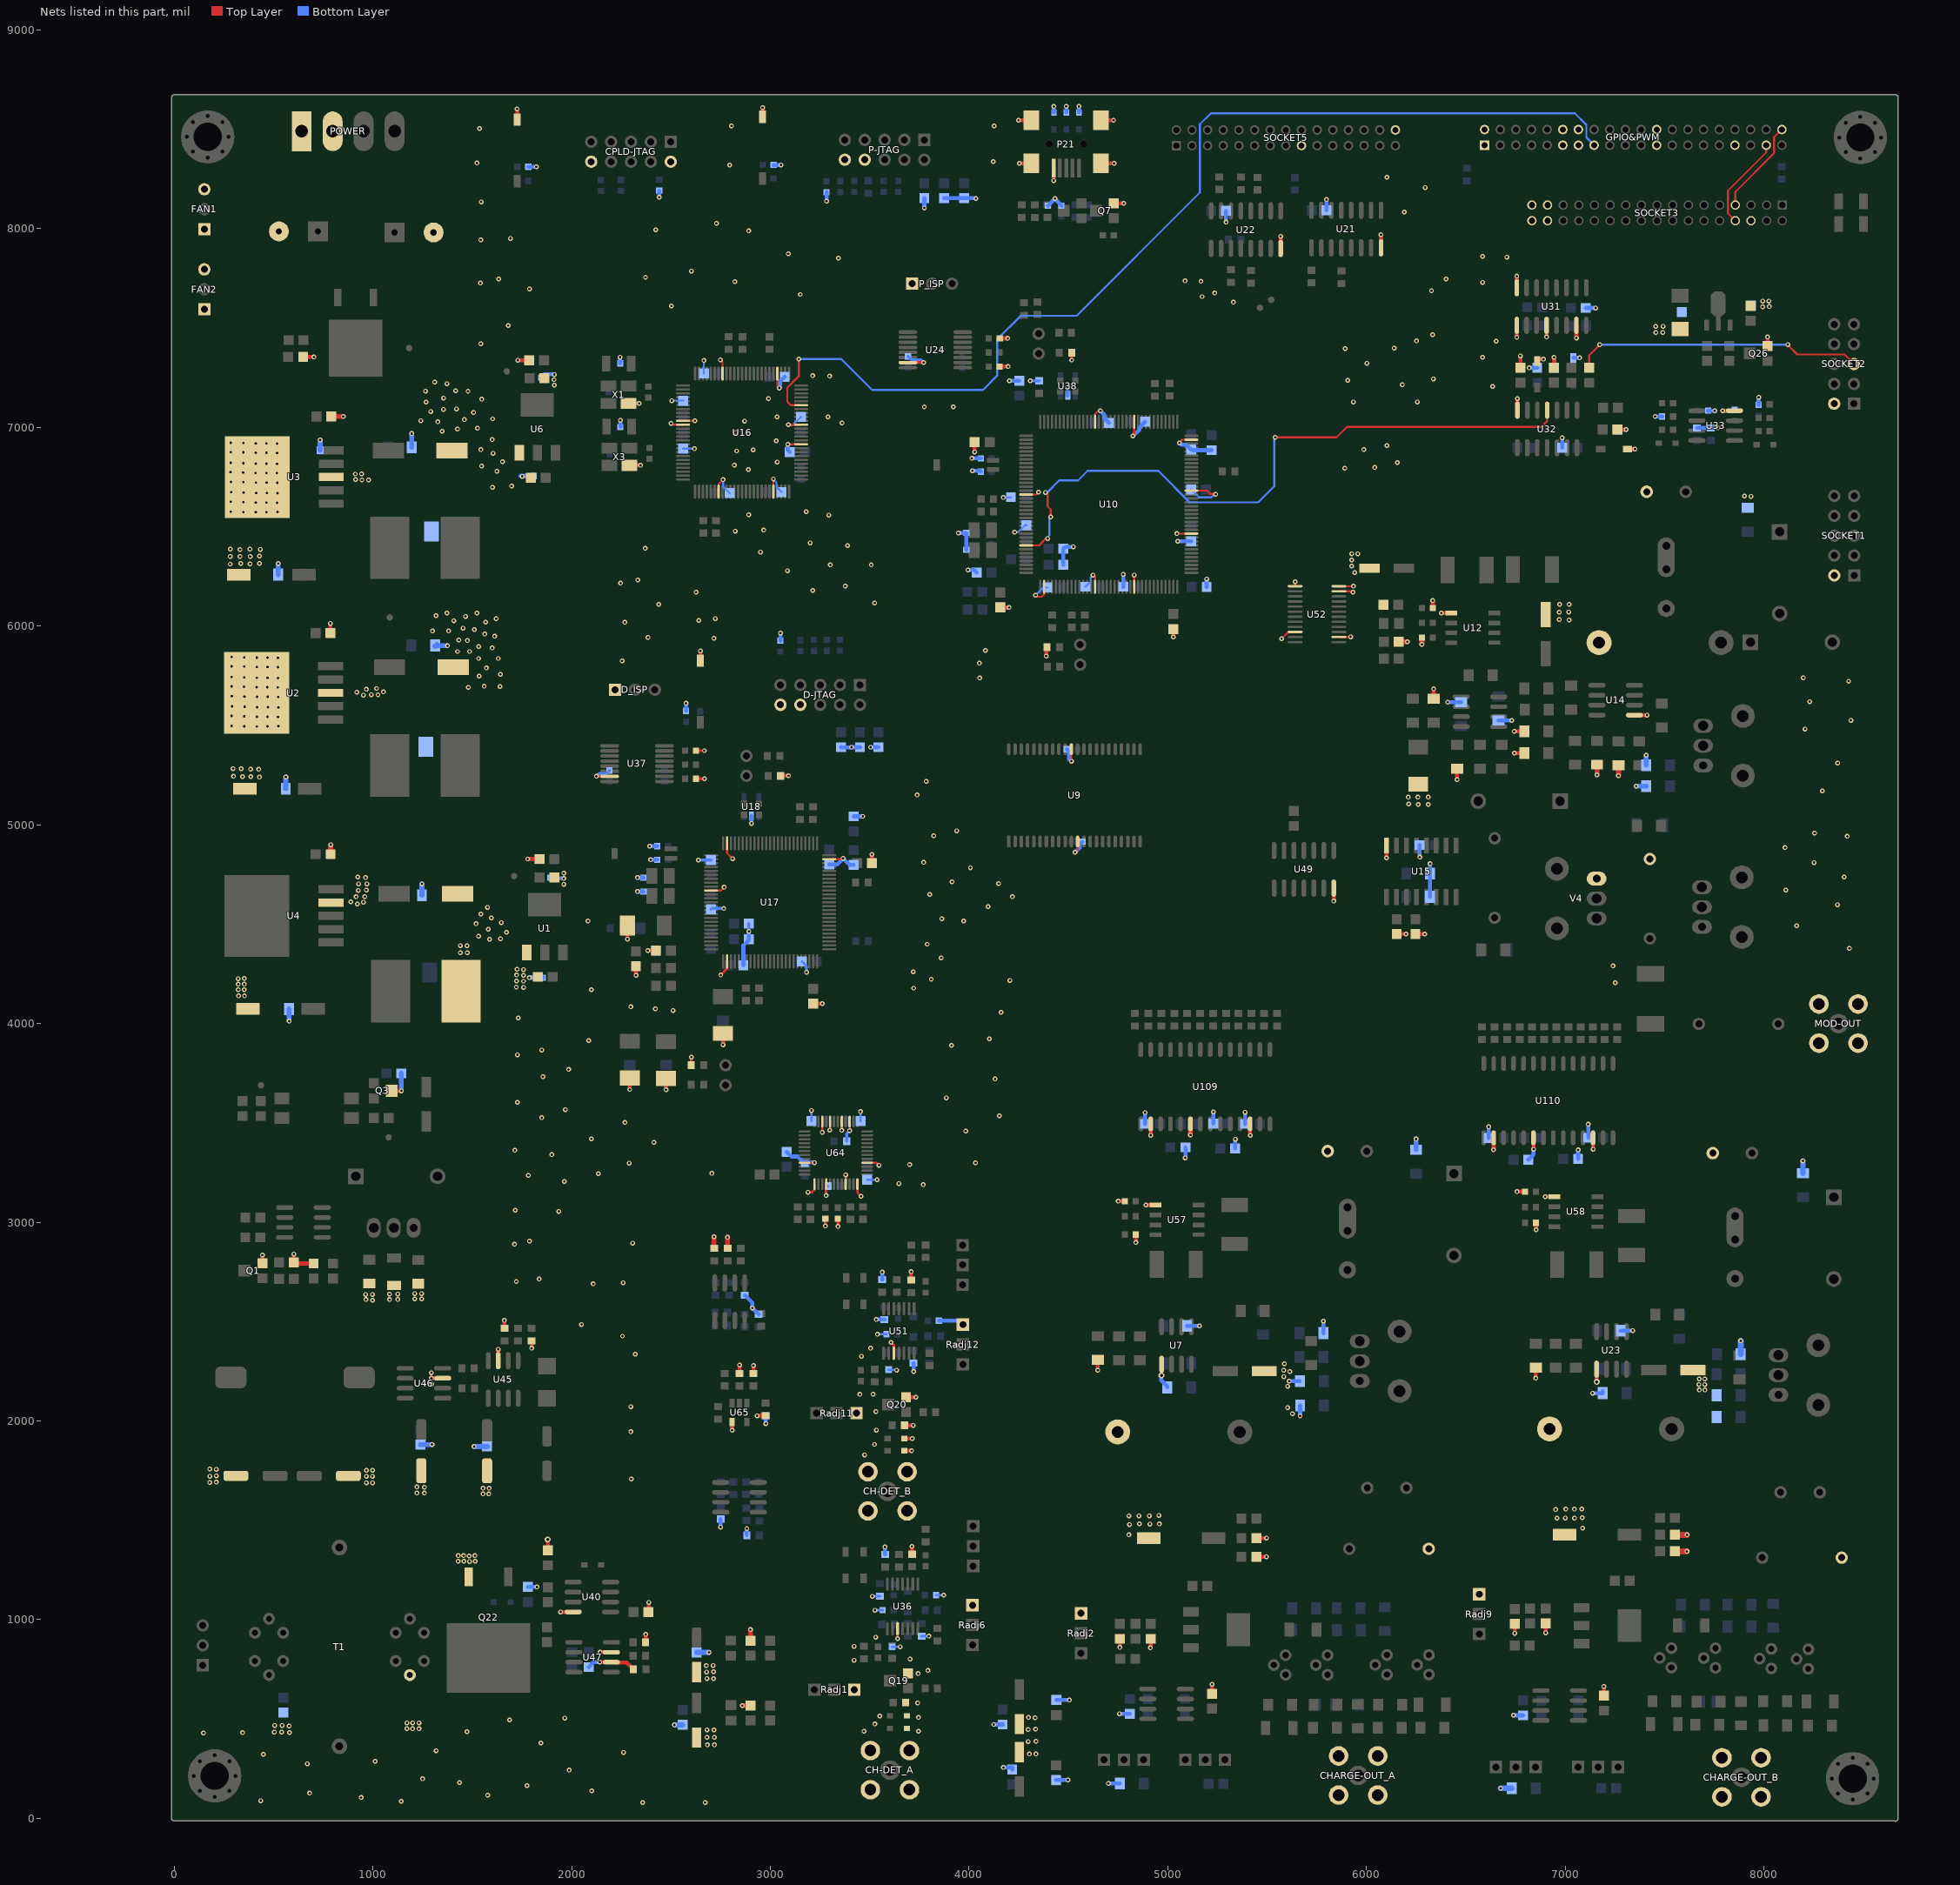
[diagram p0: the nets of this part, all layers, seen from the top]
# Altium PCB MISC82309.PcbDoc (part 8 of 14)
Units mil, origin at the board's own origin, x right, y up, seen from the top; angles counter-clockwise.
Board outline 8687.03 x 8687.86 mil, 4 copper layers (Top Layer, GND, POWER, Bottom Layer); 747 components, 583 nets, 2530 pads, 1834 vias.

## Via types
v1: diameter 24, hole 12, Top Layer to Bottom Layer, 1799 vias
v2: diameter 30, hole 15, Top Layer to Bottom Layer, 26 vias
v3: diameter 40, hole 20, Top Layer to Bottom Layer, 9 vias

## Nets (pads, with @x,y where several pads share a name; then routed paths per layer and width w, separated by ;. In a path a pad name is that pad's centre, name@x,y a point inside that pad or via, vN(x,y) a via of type N, cw(c..) or ccw(c..) an arc to the next point about the centre after c; other vN are vias at no path point) (continued)
GND: C1.1 C2.1 C3.2 C4.2 C5.2 C6.1 C7.1 C8.1 C9.2 C10.2 C11.2 C12.1 C13.1 C14.1 C15.2 C16.1 C18.1 C19.1 C20.1 C24.2 C25.2 C27.2 C28.2 C29.2 C31.2 C32.2 C33.1 C34.1 C35.1 C36.1 C37.1 C38.1 C39.1 C40.1 C41.1 C42.1 C45.2 C48.2 C49.2 C50.2 C51.2 C52.2 C53.2 C54.2 C55.1 C56.2 C57.2 C63.1 C64.1 C65.1 C66.1 C67.2 C68.2 C69.2 C70.1 C71.1 C72.1 C73.1 C74.1 C75.1 C78.2 C79.1 C80.1 C81.1 C82.1 C83.1 C84.1 C85.1 C86.1 C87.1 C88.1 C89.1 C90.1 C93.1 C94.1 C98.1 C99.1 C123.1 C124.1 C125.1 C126.1 C127.1 C128.1 C129.1 C130.1 C131.1 C132.1 C133.1 C134.1 C141.1 C142.1 C143.1 C146.1 C147.1 C148.1 C151.1 C153.2 C154.1 C155.2 C156.2 C157.2 C158.2 C159.1 C162.1 C164.1 C165.1 C167.2 C170.2 C171.2 C172.1 C173.1 C174.1 C175.1 C176.1 C179.1 C180.1 C181.1 C182.1 C183.1 C184.1 C188.1 C193.1 C195.1 C196.1 C197.1 C198.1 C199.1 C200.1 C201.1 C202.1 C210.1 C214.2 C215.2 C220.1 C221.1 C226.1 C227.1 C228.1 C230.1 C231.1 C232.1 C233.1 C240.1 C241.1 C242.1 C243.1 C244.1 C245.1 C246.1 C247.1 C248.1 C249.1 C250.1 C251.1 C252.1 C253.1 C254.1 C255.1 C256.2 C257.2 C263.2 C266.2 C267.2 C270.2 C271.2 C277.2 C278.2 C279.1 C280.1 C281.1 C283.2 C284.2 C285.1 C288.1 C292.2 C293.2 C317.2 C318.2 C364.1 C370.1 C373.1 C374.1 C411.1 C412.1 C413.1 C420.1 C421.1 C423.2 C424.1 C449.1 C506.2 C507.2 C599.2 CH-DET_A.2 CH-DET_B.2 CHARGE-OUT_A.M-1 CHARGE-OUT_A.M-2 CHARGE-OUT_A.M-3 CHARGE-OUT_A.M-4 CHARGE-OUT_B.M-1 CHARGE-OUT_B.M-2 CHARGE-OUT_B.M-3 CHARGE-OUT_B.M-4 CPLD-JTAG.2 CPLD-JTAG.10 CPLD_REST.1 D2.1 D3.1 D6.1 D14.1 D23.1 D24.1 D25.2 D26.1 D28.1 D29.1 D34.1 D35.1 D40.1 D46.1 D47.2 D52.1 D54.1 D55.2 D-JTAG.8 D-JTAG.10 D_ISP.1 D_REST.2 ESD23.2 ESD24.2 ESD25.2 FAN1.1 FAN1.3 FAN2.1 FAN2.3 GPIO&PWM.1 GPIO&PWM.2 GPIO&PWM.11 GPIO&PWM.12 GPIO&PWM.13 GPIO&PWM.14 GPIO&PWM.23 GPIO&PWM.24 GPIO&PWM.33 L4.2 LED1.2 LED2.2 LED3.2 LED4.1 LED5.2 LED6.2 MOD-OUT.2 P21.5 P21.6 P21.7 P21.8 P21.9 P-JTAG.8 P-JTAG.10 P_ISP.1 P_REST.2 POWER.1 POWER.2 Q1.2 Q3.3 Q7.2 Q19.2 Q20.2 Q22.3 Q26.2 R13.2 R15.2 R17.1 R22.2 R27.1 R28.1 R29.1 R33.1 R34.2 R39.1 R46.2 R48.1 R61.2 R62.2 R64.2 R65.2 R68.1 R74.1 R76.1 R79.1 R84.1 R85.1 R151.1 R157.1 R158.1 R168.1 R174.2 R190.1 R192.1 R194.1 R197.1 R217.2 R220.2 R221.1 R222.2 R269.2 R275.1 R286.1 R287.1 R292.1 R293.2 R294.1 R295.2 R313.1 R314.2 R315.1 R316.1 R318.2 R326.1 R328.1 R330.1 R333.1 R343.1 R374.2 R411.2 R417.2 R495.1 R496.1 R517.2 R521.2 R545.1 R546.1 R555.1 R591.1 R595.1 R599.1 Radj1.1 Radj2.3 Radj6.1 Radj9.3 Radj11.1 Radj12.1 SOCKET1.2 SOCKET2.2 SOCKET3.6 SOCKET3.31 SOCKET3.32 SOCKET3.33 SOCKET3.34 SOCKET5.17 SOCKET5.30 T1.3 TC2.1 TC3.1 U1.1 U2.3 U2.6 U3.3 U3.6 U4.4 U6.1 U7.5 U9.12 U9.34 U10.16 U10.38 U10.51 U10.61 U10.83 U10.94 U10.107 U10.120 U10.130 U12.1 U14.5 U15.16 U16.10 U16.11 U16.32 U16.46 U16.60 U16.65 U16.79 U16.93 U17.10 U17.27 U17.74 U17.99 U18.2 U21.8 U22.8 U23.5 U24.15 U31.8 U31.9 U31.12 U31.15 U32.7 U33.4 U36.3 U37.15 U38.2 U40.4 U45.3 U46.3 U47.2 U47.3 U49.7 U51.3 U52.2 U52.11 U52.12 U52.13 U52.22 U57.1 U58.1 U64.1 U64.4 U64.9 U64.12 U64.16 U64.27 U64.29 U64.32 U64.34 U64.45 U65.4 U109.16 U109.20 U109.26 U110.16 U110.20 U110.26 V1.1 V4.3 X1.2 X3.2 | length 17920.4
  Top Layer w10: v1(2501,7020) 2507.63,7013.37 U16.11@2560.76,7013.37 ; U16.10@2560.76,7033.06 v1(2620.06,7033.06) ; U17.10@2701.76,4669.06 2751.06,4669.06 v1(2768,4686) ; U16.32@2739.89,6676.76 2739.89,6714.89 v1(2762,6737) ; v1(2749,7339) 2759.57,7328.43 U16.93@2759.57,7271.24 ; U17.99@2782.46,4907.24 2782.46,4857.54 v1(2810,4830) ; U16.46@3015.48,6676.76 v1(3015.48,6740.48) ; U16.79@3035.17,7271.24 3035.17,7206.83 3044,7198 v1(3045,7198) ; v1(3088.06,6914.94) U16.60@3155.24,6914.94 ; v1(3090.63,7013.37) U16.65@3155.24,7013.37 ; U64.45@3172.52,3299.79 v1(3221.79,3299.79) ; U17.74@3296.24,4826.54 v1@3361.54,4826.54 ; U10.16@4287.65,6662.21 4338.21,6662.21 v1(4350,6674) ; v1(4335,6155) 4342,6148 4365,6148 4378.2,6161.2 U10.38@4378.2,6197.65 ; v1(4514.96,5320.04) U9.34@4514.96,5380.57 ; v1(4533,4862) 4532,4862 4546.46,4876.46 U9.12@4546.46,4916 ; v1(4624,6257) 4634.1,6246.9 U10.51@4634.1,6197.65 ; U10.130@4634.1,7028.35 4634.1,7067.1 4650,7083 v1(4661,7083) ; v1(4825,6957) 4826,6957 4831,6962 4830.95,6962.05 U10.120@4830.95,7028.35 ; U10.61@4830.95,6197.65 v1(4830.95,6256.95) ; v1(5046.36,6465.36) U10.83@5118.35,6465.36 ; v1@5059,6924 5072.8,6937.8 U10.107@5118.35,6937.8 ; U10.94@5118.35,6681.9 5196.1,6681.9 5212,6666 v1@5235,6666 ; v1(5573,5937) 5606.43,5970.43 U52.22@5640.76,5970.43 ; U52.13@5640.76,6200.75 v1(5640.76,6222.76) ; U52.2@5861.24,5944.84 5920.16,5944.84 5920,5945 v1(5920,5946) ; U52.11@5861.24,6175.16 5927.84,6175.16 v1(5932,6171) ; U52.12@5861.24,6200.75 v1(5933.75,6200.75)
  Top Layer w11: v1(3190,3151) 3211,3151 3221.73,3161.73 U64.1@3221.73,3191.52 ; v1(3261.1,3452.1) U64.34@3261.1,3506.48 ; v1(3280.79,3134.21) U64.4@3280.79,3191.52 ; v1(3299,3463) 3300,3462 3300.47,3462.47 U64.32@3300.47,3506.48 ; v1(3359.53,3462.47) U64.29@3359.53,3506.48 ; U64.9@3379.21,3191.52 v1(3379.21,3238.79) ; v1(3398.9,3461.1) U64.27@3398.9,3506.48 ; U64.12@3438.27,3191.52 3438.27,3148.73 v1(3456,3131) ; U64.16@3487.48,3299.79 3534.21,3299.79 v1(3547,3287)
  Top Layer w12: v1(2750.64,4244) 2782.46,4275.82 U17.27@2782.46,4312.76 ; v1(3608,2395) 3621.41,2381.59 U51.3@3621.41,2340.8 ; v1(3640,905) 3640.41,905.41 U36.3@3640.41,954.8 ; v1@3709,2749 3710,2750 v1(3709,2751)
  Top Layer w15: v1(2125.02,5244.02) U37.15@2191.2,5244.02 ; R62.2@2602.5,3791 v1(2602.5,3830.5) ; C179.1@2626.5,5232 v1(2669,5232) ; C180.1@2626.5,5373 v1(2668,5373) ; v1(3277,2981) C506.2@3277,3018.5 ; v1(3340,2979) C507.2@3340,3018.5
  Top Layer w16: U24.15@3692.2,7326.02 v1(3771.98,7326.02) ; v1(4516.5,7338.5) R64.2@4516.5,7375
  Top Layer w20: Q1.2@444,2793 v1(444,2835) ; R13.2@602.5,2798 v1(602.5,2840.5) ; R13.2@613.5,2792.5 C193.1@702,2792.5 ; LED5.2@649.5,7354 v1(704,7354) ; v1(786,6014) 786.5,6013.5 LED2.2@786.5,5965 ; Q3.3@1095,3661 v1(1144,3661) ; v1(1295,2215) U46.3@1351.49,2215 ; U45.3@1631,2303.49 v1(1631,2361) ; C226.1@1662,2466.5 v1(1662,2506) ; v1(1726,8602) 1727,8601 CPLD_REST.1@1727,8549 ; v1(1730,7338) LED6.2@1786.5,7338 ; v1(1779,4828) LED1.2@1838.5,4828 ; v1(1799,2366) R286.1@1799,2403.5 ; R217.2@1880,1348.5 v2(1880,1404) ; v1(1945,1039) U40.4@2007.51,1039 ; v1(2142,786) U47.2@2200.49,786 ; v1(2144,836) U47.3@2200.49,836 ; U47.2@2220,785 2276.5,785 R287.1@2310.5,751 ; v1(2281,4425) D28.1@2281,4493 ; X1.2@2287,7121 v1(2340,7121) ; X3.2@2291,6809 v1(2347,6809) ; v1(2293,3668) D29.1@2293,3726 ; v1(2324,4242) R222.2@2324,4288.5 ; C232.1@2372.5,886 2372.5,925.5 v1(2373,926) ; v1(2383,4367) C70.1@2424.5,4367 ; R220.2@2386.5,1039 2388,1040.5 v1(2388,1087) ; v1(2475,3667) D34.1@2475,3724 ; D_REST.2@2648,5826 v1(2648,5875) ; v1(2762,3893) D23.1@2762,3950 ; U65.4@2807.6,1994.76 2807.6,1953.4 v1(2808,1953) ; C420.1@2845,2239.5 v1(2845,2282) ; C421.1@2915,2239.5 v1(2915,2279) ; v1(2933,2026) 2933.5,2026.5 C423.2@2977,2026.5 ; v1(2961,8609) 2961.17,8608.83 P_REST.2@2961.17,8563 ; R61.2@3051.5,5247 v1(3092,5247) ; C256.2@3216,4100.5 v1(3261.5,4100.5) ; C257.2@3511.5,4807 v1(3511.5,4851.5) ; v1(3635,2256) v1@3635.5,2255.5 ; D46.1@3674.32,1850 v1(3711,1850) ; D47.2@3674.32,1912 v1(3714,1912) ; R546.1@3675.5,1978 v1(3719,1978) ; Q20.2@3683,2119.5 3731.5,2119.5 v1(3732,2119) ; R330.1@3709,2708.5 v1@3709,2749 ; R194.1@3713,1329.5 v1(3713,1369) ; v1(4028.5,6876.5) C128.1@4028.5,6926 ; C93.1@4153.5,7306 v1(4197,7306) ; C94.1@4154.5,7448 v1(4195,7448) ; C36.1@4157,6093.5 4196.5,6093.5 v1@4198,6092 ; v1(4249.11,8545.11) P21.8@4313.8,8545.11 ; v1(4253.57,8328.57) P21.9@4313.8,8328.57 ; v1(4388,5849) 4388,5890.5 R65.2@4392.5,5895 ; v1(4426.01,8242.01) P21.5@4426.01,8304.95 ; v1(4648,2255) R17.1@4648,2307 ; P21.7@4664.2,8328.57 v1(4729.43,8328.57) ; P21.6@4664.2,8545.11 v1(4727.11,8545.11) ; Q7.2@4729,8127.5 v1(4778.5,8127.5) ; v1(4751,3106) C280.1@4784,3106 ; v1(4759,860) R22.2@4759,903.5 ; v1(4839,2898) R151.1@4839,2938 ; v1(4890,3087) U57.1@4939,3087 ; v1(4913,858) 4914,859 R33.1@4914,903.5 ; v1(4914,3438) U109.16@4914,3494.99 ; v2(4968,2229) 4969,2230 U7.5@4969,2285.51 ; v1(5028,5945) C215.2@5028,5985.5 ; R48.1@5223,626.5 v1(5223,675) ; U109.26@5414,3494.99 5414,3438 v1(5415,3437) ; C157.2@5445.5,1317 v1(5496,1317) ; R46.2@5445.5,1411 v1(5497,1411) ; U22.8@5568,7900.51 v1(5568,7962) ; v1(5835,4616) U49.7@5835,4681.51 ; U21.8@6073,7903.51 v1(6073,7970) ; v1(6101,4834) U15.16@6101,4896 ; C318.2@6152,4450.5 v1(6199.5,4450.5) ; C317.2@6246,4450.5 v1(6293.5,4450.5) ; R68.1@6333.5,6091 v1(6333.5,6128.5) ; C45.2@6338,5634 v1(6338,5684) ; v1(6376,6066) U12.1@6427,6066 ; v1(6456,5227) R79.1@6456,5282 ; v1(6639,3365) 6640,3366 U110.16@6640,3424.99 ; v1(6743,5470) R76.1@6795,5470 ; v1(6744,5361) C49.2@6795,5361 ; v1(6746,932) R314.2@6746,979.5 ; v1(6756,7453) U31.9@6756,7513.51 ; U31.8@6756,7702.49 v1(6756,7761) ; v1(6757,3154) C281.1@6797.5,3154 ; U32.7@6759,7086.49 v1(6759,7145) ; C162.1@6774,7299.5 v1(6774,7360) ; U110.20@6840,3424.99 6840,3369 v1(6841,3368) ; v1(6852,2215) 6851,2215 6850,2216 6852,2218 R221.1@6852,2269 ; R343.1@6852.5,2997 6852.5,2962.5 v1(6853,2962) ; D24.1@6859,7333.93 6868.07,7343 v1(6891,7343) ; v1(6899,3128) U58.1@6946,3128 ; v1(6901,934) R316.1@6901,980.5 ; v1(6906,7455) U31.12@6906,7513.51 ; C373.1@6943,7300.5 6943,7352 v1(6944,7353) ; v1(7056,7450) U31.15@7056,7513.51 ; U110.26@7140,3424.99 7140,3369 v1(7141,3368) ; v2(7158,2197) U23.5@7158,2260.51 ; R292.1@7194,617.5 v1(7194,664) ; R496.1@7262.5,6989 v1(7306,6989) ; D52.1@7312.93,6891 v1(7351,6891) ; U14.5@7348.49,5552 v1(7412,5552) ; v1(7792,7084) U33.4@7851.49,7084 ; Q26.2@8018,7409 v1(8018,7455)
  Top Layer w25: LED4.1@787.5,4852 v1@787.5,4898.5 ; LED3.2@790.5,7055 v1@850,7055 ; C599.2@2717,2869.5 v1(2717,2927) ; R599.1@2785,2869.5 v1(2785,2924) ; v1(2859.5,567.5) C173.1@2901,567.5 ; C176.1@2900,893.5 v1(2900,950) ; v1(5114,3439) U109.20@5114,3494.99 ; C66.1@6161.5,5921 v1(6206,5921) ; v1(6278.5,5908.5) C42.1@6278.5,5942 ; v1(7160,5252) C48.2@7160,5303 ; v1(7268,5247) C51.2@7268,5300
  Top Layer w30: C277.2@7551.5,1344 v1(7612,1344) ; R295.2@7551.5,1427 v1(7613,1427)
  Bottom Layer w10: v1(2504.5,7134.5) C199.1@2561,7134.5 ; C195.1@2561,6892.5 v1(2618.5,6892.5) ; C197.1@2665.5,7271 v1(2665.5,7336.5) ; v1@2763,6733 2763,6701.5 C196.1@2795.5,6669 ; v1@3017,6736 3031,6722 3031,6699.5 C200.1@3055.5,6675 ; v1@3093,7014 3115.5,7014 C202.1@3154,7052.5 ; C412.1@3173,3296.5 3175.5,3299 v1@3219,3299 ; C247.1@3296,4800.5 C247.1@3296.5,4801 ; v1(4172,6647) 4208.5,6647 C129.1@4210.5,6649 ; v1(4230,6473) 4247,6473 4281.5,6507.5 C130.1@4289,6507.5 ; v1@4337,6158 4373,6194 C143.1@4394.5,6194 ; C142.1@4585.5,6198 4611,6223.5 4611,6242 v1@4621,6252 ; C146.1@5117.5,6688 5157.5,6648 5219.47,6648 5229.5,6658.03 5229.5,6659.5 v1@5234,6664
  Bottom Layer w11: C254.1@3207.5,3509 v1(3207.5,3562.5) ; v1@3281,3138 3281,3173.5 C413.1@3290.5,3183 ; C243.1@3453.5,3509 v1(3453.5,3556.5) ; C250.1@3488,3214.5 3538.5,3214.5 v1(3538,3214)
  Bottom Layer w12: C252.1@3158.5,4313 3182,4289.5 v1(3182,4258) ; v1(3513,1118) 3513.5,1118.5 R192.1@3552,1118.5 ; v1(3527,1048) C167.2@3565.5,1048 ; v1(3539,2436) 3540,2437 C292.2@3584.5,2437 ; C288.1@3595,2257.5 3631.5,2257.5 v1@3633,2256 ; C165.1@3613,863.5 3652.5,863.5 v1(3653,864) ; v1@3640,902 v1(3640,905) ; R197.1@3761,916.5 3796.5,916.5 v1(3797,917) ; C170.2@3833.5,1124 v1(3872,1124)
  Bottom Layer w15: v1@2127,5247 2139,5259 2176.5,5259 C181.1@2191,5273.5 ; v1(2638.5,4822.5) C87.1@2701,4822.5 ; C245.1@2701,4574.5 2705.5,4579 v1(2766,4579) ; v1@2891,4465 2892.5,4466.5 C73.1@2892.5,4503 ; v1@2892.5,4462 v1(2892.5,4463.5) ; C411.1@3384.5,3408 3384.5,3445.5 v1@3397,3458
  Bottom Layer w16: C90.1@3693,7357.5 3710.5,7340 3758,7340 v1(3771.98,7326.02) ; v1(4307.5,7234.5) R275.1@4353,7234.5
  Bottom Layer w20: C184.1@1780,1164.5 v1(1826.5,1164.5) ; C244.1@1782.5,8311 v1(1823,8311) ; C20.1@1846.5,7251 1862.5,7267 v1@1913,7267 ; C7.1@1893.5,4734 1896.5,4731 v1@1961,4731 ; C233.1@2086,761.5 2110.5,786 v1@2139,786 ; C34.1@2244.5,7322 v1(2244.5,7353.5) ; C75.1@2245.5,7002 v1(2245.5,7035.5) ; v1(2331,4734) C80.1@2361.5,4734 ; v1(2332,4664) C81.1@2362.5,4664 ; v1(2383,4367) 2419,4367 C71.1@2422,4364 ; v1(2393,4893) C84.1@2431.5,4893 ; v1(2398,4824) C85.1@2431.5,4824 ; v1(2441,8158) R294.1@2441,8191.5 ; C74.1@2576,5573.5 v1(2576,5612) ; v1(2750,1466) R517.2@2750,1506.5 ; C251.1@2864.5,4293 2864.5,4392.5 2892,4420 v1@2892,4462 ; R417.2@2872,2632.5 2909,2595.5 2909,2570 v1@2910,2569 ; R521.2@2881.5,1425 2881.5,1457.5 v1(2882,1458) ; v1(2905,5007) U18.2@2905,5044.76 ; v1(2909,2568) 2912.5,2564.5 2914,2564.5 R411.2@2942,2536.5 ; C424.1@2977,2026.5 2977,1988 v1(2978,1987) ; C39.1@3016.5,8321 v1(3054,8321) ; v1@3046,7200 3050,7204 3050,7231.5 C201.1@3072.5,7254 ; R595.1@3051,5926.5 v1(3051,5965) ; C86.1@3082,3354.5 3105.5,3331 3136,3331 3166,3301 v1@3222,3301 ; v1@3087,6913 3087,6887.5 C198.1@3098.5,6876 ; v1(3283,8139) R591.1@3283,8183.5 ; C247.1@3296.5,4801 3337,4801 3366,4830 3367,4830 3398.5,4798.5 C253.1@3420,4798.5 ; C249.1@3356,5390.5 3356.5,5390 v1@3404,5390 ; v1(3408.5,5390.5) C255.1@3451,5390.5 ; C88.1@3419,5042.5 v1(3465.5,5042.5) ; v1(3504.5,5390.5) C242.1@3545,5390.5 ; v1(3533.5,2510.5) R328.1@3574,2510.5 ; R326.1@3563,2711.5 v1(3563,2749) ; R190.1@3577,1328.5 v1(3577,1366) ; v1(3721,2249) R333.1@3721,2290.5 ; v1(3775,8104) C131.1@3775,8153.5 ; C293.2@3848.5,2505 Radj12.1@3941,2505 ; C132.1@3874,8153.5 3965.5,8153.5 3966,8153 4033,8153 v1(4034,8152) ; v1(3946,6469) C40.1@3986.5,6469 ; C40.1@3982,6464 3986.5,6459.5 C41.1@3986.5,6384 ; v1(3994,6282) 4025.01,6282 R269.2@4038.5,6268.51 ; v1(4014,6844) C98.1@4059.5,6844 ; v1(4017,6782) 4054.5,6782 C99.1@4059.5,6777 C99.1@4055.5,6781 ; v1(4124.5,472.5) C155.2@4169,472.5 ; C35.1@4157,6093.5 v1(4201.5,6093.5) ; v1(4173,256) 4174,257 4217,257 C156.2@4217,246.5 ; v1(4202.5,7234.5) C127.1@4253,7234.5 ; C241.1@4397,8115.5 v1(4433,8151.5) ; ESD23.2@4427,8584.32 v1(4427,8615) ; v1@4435,8147 4465,8117 C240.1@4465,8115.5 ; C79.1@4438,193.5 v1(4497.5,193.5) ; C89.1@4439,595.5 v1(4504.5,595.5) ; C38.1@4474.5,6309 C37.1@4474.5,6373.5 ; C37.1@4474.5,6389 4484.51,6399 v1(4525,6399) ; ESD25.2@4489,8584.32 v1(4489,8616) ; C148.1@4491.5,5381 4503,5369.5 4503,5331 v1@4513,5321 ; U38.2@4497,7160.76 v1(4497,7203) ; v1@4536,4864 4557,4885 4557,4901.5 C147.1@4570.5,4915 ; ESD24.2@4553,8584.32 v1(4553,8615) ; v1@4664,7080 4680,7064 4680,7046.5 C126.1@4703.5,7023 ; v1(4701,176) C69.2@4759,176 ; v1(4757,527) 4757.5,526.5 R27.1@4809,526.5 ; C134.1@4775.5,6198 v1(4775.5,6260.5) ; v1@4830,6960 4857,6987 4857,6998.5 C125.1@4886.5,7028 ; C32.2@4885.5,3495 4885.5,3551.5 v1(4886,3552) ; v2@4968,2226 4967,2225 4967,2205 4997,2175 C24.2@4997,2169 ; v1(5049.5,6426.5) C123.1@5117,6426.5 ; v1@5059,6920 5061,6920 5069,6912 5094,6912 5116.5,6889.5 C124.1@5118,6889.5 ; v1(5088,3324) 5088.5,3324.5 R34.2@5088.5,3377 ; C25.2@5097,2479 v1(5159,2479) ; C124.1@5126.5,6885.5 C214.2@5221,6885.5 ; C141.1@5195.5,6197 v1(5195.5,6237.5) ; C246.1@5228.5,3496 5228.5,3554.5 v1(5229,3555) ; v1(5293.5,8032.5) C82.1@5293.5,8090 ; C33.1@5338.5,3371 5338.5,3416.5 v1(5340,3418) ; C31.2@5388.5,3495 5388.5,3553.5 v1(5389,3554) ; v1(5611,2201) R29.1@5665,2201 ; v1(5666,2025) R28.1@5666,2078 ; C27.2@5783,2442 v1(5783,2503) ; C83.1@5798.5,8092 v1(5798.5,8146.5) ; C56.2@6267.5,4898 6267.5,4837.5 v1(6268,4837) ; C63.1@6320,4638 C57.2@6320,4742 ; C57.2@6320,4755 v1(6320,4804) ; v1(6408,5617) C53.2@6476,5617 ; v1(6615,3480) 6615.5,3479.5 C284.2@6615.5,3424 ; C50.2@6664,5525 v1(6731,5525) ; v1(6740,519) 6740.5,518.5 R315.1@6788,518.5 ; R318.2@6814.5,3315 6837,3337.5 6837,3339 6841,3343 v1@6841,3367 ; v1(6818.5,7299.5) R168.1@6859,7299.5 ; R495.1@6944,7299.5 v1(6944,7353) ; v1(6984,6948) 6985.5,6946.5 C154.1@6985.5,6897 ; D54.1@7041,7349.93 v1(7071.93,7349.93) ; C285.1@7064.5,3318 7064.5,3363.5 v1(7065,3364) ; C151.1@7103.5,7601 v1(7153,7601) ; v1(7115,3493) 7115.5,3492.5 C283.2@7115.5,3425 ; v1(7137,2140) C270.2@7188,2140 C270.2@7188,2150 ; C374.1@7262.5,6989 7263.5,6988 v1@7306,6988 ; C271.2@7279,2455 v1(7339,2455) ; v1(7452,7055) R174.2@7487.5,7055 ; C370.1@7663,6997.5 v1(7768.5,6997.5) ; C164.1@7718.5,7084 v1(7752,7084) ; v1(7792,7084) C364.1@7846,7084 ; R374.2@7973,7112.5 v1(7973,7151)
  Bottom Layer w25: C14.1@524,6259 v1(524,6315) ; C8.1@562,5181 v1(562,5241) ; v1@579,4014 C16.1@579,4073 ; v1(735,6937) 735,6885.5 R555.1@735.5,6885 ; v1@1143.5,3662.5 R15.2@1143.5,3749 ; C15.2@1196,6900 v1(1196,6969) ; C231.1@1239,1881.5 v1(1297.5,1881.5) ; C13.1@1247,4645 v1(1247,4703) ; C5.2@1313,5898 C5.2@1322,5907 ; C5.2@1322,5901 v1@1373,5901 ; v1(1509.5,1871.5) C183.1@1575,1871.5 ; v1@1746,6755 C19.1@1808.5,6755 ; v1(1788,4231) C6.1@1855,4231 ; v1(2517.5,470.5) C172.1@2559,470.5 ; C175.1@2629,835.5 v1(2691.5,835.5) ; R39.1@6249,3365 v1(6249,3419) ; v1(7357,5195) R84.1@7407,5195 ; R85.1@7407,5300 v1(7407,5350) ; R313.1@8196,3246 v1(8196,3309)
  Bottom Layer w30: v1(6675,152) C278.2@6731,152 ; C263.2@7883,2336 v1(7883,2403)
  other v1: 2358,80 2672,80 1143,86 436,89 941,105 1578,117 682,127 2101,139 1776,165 1436,180 1250,199 1988,243 670,275 1012,287 449,322 4303,324 4336,324 2261,332 1319,341 2683,370 2719,370 1846,379 4298,387 4337,388 2681,408 2718,408 148,430 345,431 580,432 505,434 541,434 1474,436 3471,439 3746,439 2717,445 2681,446 4298,447 4335,449 1200,451 1232,451 1171,452 579,465 506,468 543,468 3526,475 1171,481 1201,481 1232,481 1688,496 1966,505 4333,506 3746,508 4299,508 3551,515 3742,581 2715,703 2681,704 3744,729 2680,737 2715,738 3793,744 2678,769 2712,770 3421,796 3703,802 3422,866 3530,912 1487,1293 1429,1294 1458,1294 1515,1294 1485,1321 1430,1322 1457,1322 1514,1322 4804,1427 7087,1461 4808,1479 4910,1481 4957,1482 4857,1483 6959,1511 7047,1511 7000,1512 7085,1513 4804,1523 4855,1523 4907,1523 4955,1525 6952,1554 7003,1556 7046,1556 7083,1557 1554,1633 1584,1633 1222,1637 1260,1637 1555,1661 1585,1661 1260,1666 1222,1668 967,1689 999,1689 179,1691 212,1692 2300,1708 180,1722 967,1722 998,1722 212,1724 968,1752 999,1752 212,1757 179,1758 3475,1829 3524,1882 2298,1946 3534,1954 5627,2036 3532,2047 5603,2067 2298,2072 3451,2134 3517,2135 7675,2156 7703,2156 5603,2175 7673,2184 7702,2184 1296,2185 7674,2211 7702,2211 5584,2223 1295,2243 5614,2249 5583,2255 5587,2288 3459,2326 2321,2336 3505,2366 2256,2427 2050,2486 999,2608 965,2611 1085,2611 1126,2611 1211,2614 1246,2614 964,2637 998,2637 1085,2638 1125,2639 1211,2641 1245,2641 2109,2690 2259,2696 1722,2702 1837,2714 1713,2889 2308,2895 1788,2905 1936,3055 1716,3061 3769,3189 3647,3195 1964,3205 1783,3236 2135,3244 2706,3246 3701,3290 2290,3298 4033,3299 1900,3340 1714,3362 2414,3402 2099,3420 3983,3459 2269,3502 1850,3526 4152,3536 1969,3567 1727,3604 3885,3626 4131,3721 1856,3733 1985,3769 1727,3843 1850,3867 3912,3890 2086,3914 4102,3923 579,4012 1732,4028 4161,4056 2510,4066 2422,4074 2298,4084 324,4139 354,4139 323,4170 353,4170 2099,4170 3722,4178 1759,4182 1722,4184 323,4198 353,4198 7252,4205 1758,4213 1723,4214 4206,4217 3810,4223 322,4226 353,4227 1758,4242 1724,4244 3719,4260 1758,4272 1726,4273 7240,4290 3860,4330 1440,4356 1475,4356 8430,4378 1474,4391 1440,4392 3790,4399 1587,4424 1643,4426 1532,4440 1673,4459 1581,4475 8164,4492 1519,4502 1646,4508 2083,4516 3973,4516 3863,4527 1596,4531 1544,4551 1577,4585 4096,4588 8370,4598 922,4601 953,4611 889,4612 916,4638 4218,4638 960,4639 3802,4650 927,4670 967,4671 8110,4672 1961,4701 929,4703 970,4703 4149,4704 3915,4713 1961,4730 964,4734 924,4737 8403,4737 1961,4757 4007,4784 8252,4810 3772,4811 3366,4831 8106,4885 788,4900 8419,4942 3823,4945 8255,4958 3938,4970 6260,5103 6311,5103 6212,5105 6210,5139 6259,5139 6311,5139 3739,5150 8294,5171 3784,5219 429,5240 344,5243 386,5243 299,5244 426,5279 385,5280 338,5282 297,5283 8371,5311 8207,5482 416,5495 353,5496 470,5496 525,5497 290,5498 8437,5526 523,5543 416,5544 470,5544 353,5546 290,5548 525,5591 418,5592 472,5592 355,5594 292,5596 8230,5620 524,5643 417,5644 471,5644 354,5646 291,5648 953,5653 1026,5654 992,5655 919,5667 1053,5669 967,5682 1019,5686 522,5692 1481,5692 415,5693 469,5693 352,5695 1640,5696 289,5697 1560,5697 8426,5723 523,5739 4053,5739 416,5740 470,5740 8198,5740 353,5742 290,5744 1535,5748 1642,5757 1571,5789 523,5793 416,5794 470,5794 353,5796 290,5798 4052,5813 2254,5825 1532,5837 1631,5837 523,5840 416,5841 470,5841 353,5843 290,5845 1426,5872 1487,5872 4082,5877 1600,5890 1533,5897 1376,5901 1476,5927 1433,5930 2716,5939 2385,5943 1613,5949 1563,5960 1300,5975 1382,5975 1511,5982 1454,5990 2268,6019 1568,6020 1407,6027 2640,6029 7019,6031 6970,6033 1621,6037 2723,6038 1466,6049 1318,6053 1373,6066 1524,6066 6970,6070 7018,6071 2439,6109 6972,6109 7019,6110 3525,6116 2626,6171 3214,6179 3377,6202 2247,6216 2333,6232 5941,6269 3086,6279 5925,6302 3302,6308 3508,6308 282,6312 382,6313 335,6315 430,6315 5925,6333 282,6350 332,6350 383,6350 429,6353 5926,6364 5956,6364 2951,6373 332,6385 434,6386 382,6387 283,6388 2370,6391 3389,6405 3201,6419 2823,6478 2967,6483 3295,6559 2891,6560 411,6573 348,6574 465,6574 520,6575 285,6576 3181,6576 518,6621 411,6622 465,6622 348,6624 285,6626 7935,6653 7902,6655 5241,6663 520,6669 413,6670 467,6670 350,6672 287,6674 1602,6698 1698,6705 519,6721 412,6722 466,6722 349,6724 286,6726 945,6736 978,6736 913,6738 1751,6754 912,6765 943,6766 517,6770 410,6771 464,6771 347,6773 284,6775 1624,6779 2890,6788 5891,6795 6041,6798 1547,6805 2819,6810 518,6817 411,6818 465,6818 348,6820 285,6822 6155,6823 3035,6826 1652,6827 1605,6870 518,6871 411,6872 465,6872 348,6874 285,6876 2831,6881 2914,6887 1544,6888 5986,6889 6103,6908 518,6918 411,6919 465,6919 348,6921 5058.39,6921.61 285,6923 3030,6932 1600,6938 2826,6975 1349,6981 1426,6991 1527,6996 3361,7022 1327,7028 2871,7032 1241,7034 1460,7039 1603,7043 3034,7053 3290,7053 851,7055 1507,7075 1291,7080 1355,7091 1421,7093 3775,7103 3921,7103 1268,7127 5934,7128 6256,7128 1548,7142 2991,7145 1356,7148 1479,7182 1265,7183 1417,7184 6634,7206 1913,7213 6180,7215 1373,7220 1311,7228 5906,7237 1912,7240 6336,7244 3298,7258 3213,7260 1913,7266 6002,7323 6584,7353 5893,7397 6139,7399 1543,7421 6652,7434 6251,7435 6332,7467 7456,7477 7491,7477 7455,7508 7492,7509 1681,7513 7993,7607 8026,7608 2502,7611 5330,7630 7994,7636 8025,7636 5173,7658 3151,7669 5237,7676 6327,7688 1788,7696 1541,7726 6584,7730 2821,7733 5167,7735 5087,7737 1633,7747 6400,7747 2372,7755 2603,7787 3343,7852 6706,7857 6584,7861 3090,7874 1543,7944 1692,7951 2891,7989 2423,7994 2729,8027 6190,8084 1545,8135 6295,8207 6103,8259 2796,8320 1524,8330 4122,8338 1537,8504 2805,8517 4126,8517
GPIO9: GPIO&PWM.40 SOCKET3.7 | length 476.8
  Top Layer w10: SOCKET3.7@7855.78,8119 7855.78,8184.78 8051,8380 8051,8459.68 GPIO&PWM.40@8090.06,8498.74
GPIO10: GPIO&PWM.37 SOCKET3.8 | length 474.6
  Top Layer w10: SOCKET3.8@7855.78,8040.26 7819,8077.04 7819,8191 8011.32,8383.32 GPIO&PWM.37@8011.32,8420
HALL-SINGLE: R491.1 SOCKET2.5 | length 1461.2
  Top Layer w10: R491.1@7120,7299.5 7120,7363 v1@7173.5,7416.5 ; v1(8120,7417) 8119,7416 8168,7367 8210,7367 8355,7367 8405,7367 SOCKET2.5@8453,7319
  Bottom Layer w10: v1(7174,7416) 8119,7416 v1(8120,7417)
HALL-SWITCH: U10.29 U32.4 | length 3380.4
  Top Layer w10: U10.29@4287.65,6406.31 4352.31,6406.31 4391.5,6445.5 v1(4396,6441) ; v1(4385,6673) 4385,6674 4396,6663 4396,6602 4411,6587 v1(4411,6550) ; v1(5541,6950) 5849,6950 5902,7003 6880,7003 6909,7032 U32.4@6909,7086.49
  Bottom Layer w10: v1(4385,6673) 4394,6673 4454,6733 4549,6733 4597,6781 4952,6781 5110,6623 5455,6623 5536,6704 5536,6945 v1(5541,6950) ; v1(4396,6441) 4391.5,6445.5 4404,6458 4404,6543 v1(4411,6550)
HEAD-OPEN: GPIO&PWM.15 U16.70 | length 5370.1
  Top Layer w10: v1(3143,7344) 3143,7257 3086,7200 3086,7129 3103.2,7111.8 U16.70@3155.24,7111.8
  Bottom Layer w10: v1(3143,7344) 3357,7344 3512,7189 4070,7189 4141,7260 4141,7442 4261,7562 4542,7562 5162,8182 5162,8526 5217,8581 7048,8581 7106,8523 7106,8459.18 GPIO&PWM.15@7145.18,8420